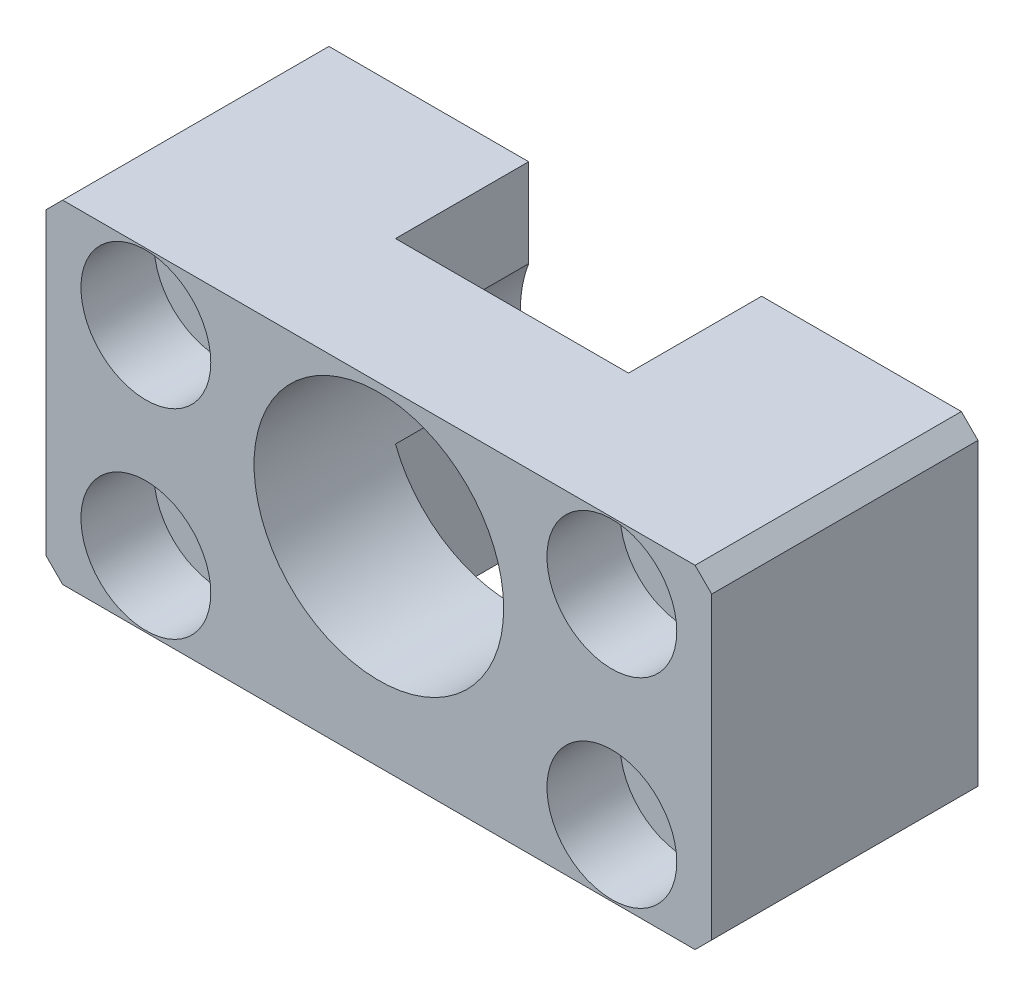
from build123d import *

# Parameters (mm, degrees)
SKETCH_1_W                   = 40
SKETCH_1_H                   = 20
EXTRUDE_1_DEPTH              = 8
CHAMFER_1_SIZE               = 1
HOLE_WIZARD_15_0_15_1_D      = 15
HOLE_WIZARD_15_0_15_1_DEPTH  = 20
CUT_EXTRUDE_2_DEPTH          = 8
HOLE_WIZARD_M4_3_D           = 4.5
HOLE_WIZARD_M4_3_CBORE_D     = 7.8
HOLE_WIZARD_M4_3_CBORE_DEPTH = 4.4


with BuildPart() as part:
    # 草图1 → 凸台-拉伸1 (new, symmetric)
    with BuildSketch(Plane.XY):
        Rectangle(SKETCH_1_W, SKETCH_1_H)
    extrude(amount=EXTRUDE_1_DEPTH, both=True)

    # 倒角1
    chamfer_1_edges = [part.edges().sort_by_distance(p)[0] for p in [
        (20, -10, 0),
        (-20, -10, 0),
        (-20, 10, 0),
        (20, 10, 0),
    ]]
    chamfer(chamfer_1_edges, length=CHAMFER_1_SIZE)

    # Ø15.0 (15) 直径孔1
    with Locations(Plane.XY.offset(8)):
        with Locations((0, 2)):
            Hole(HOLE_WIZARD_15_0_15_1_D / 2, depth=HOLE_WIZARD_15_0_15_1_DEPTH)

    # 草图6 → 切除-拉伸2 (cut)
    with BuildSketch(Plane(origin=(0, 0, -8), x_dir=(-1, 0, 0), z_dir=(0, 0, -1))):
        Polygon((-7, -14.985571338), (-7, 13.139303821), (7, 13.139303821), (7, -15.772038878), align=None)
    extrude(amount=-CUT_EXTRUDE_2_DEPTH, mode=Mode.SUBTRACT)

    # M4 六角凹头螺钉的柱形沉头孔3 (through all)
    with Locations(Plane.XY.offset(8)):
        with Locations((0, 0), (14, 6), (-14, -6), (-14, 6), (14, -6)):
            CounterBoreHole(HOLE_WIZARD_M4_3_D / 2, HOLE_WIZARD_M4_3_CBORE_D / 2, HOLE_WIZARD_M4_3_CBORE_DEPTH)


solid = part.part
